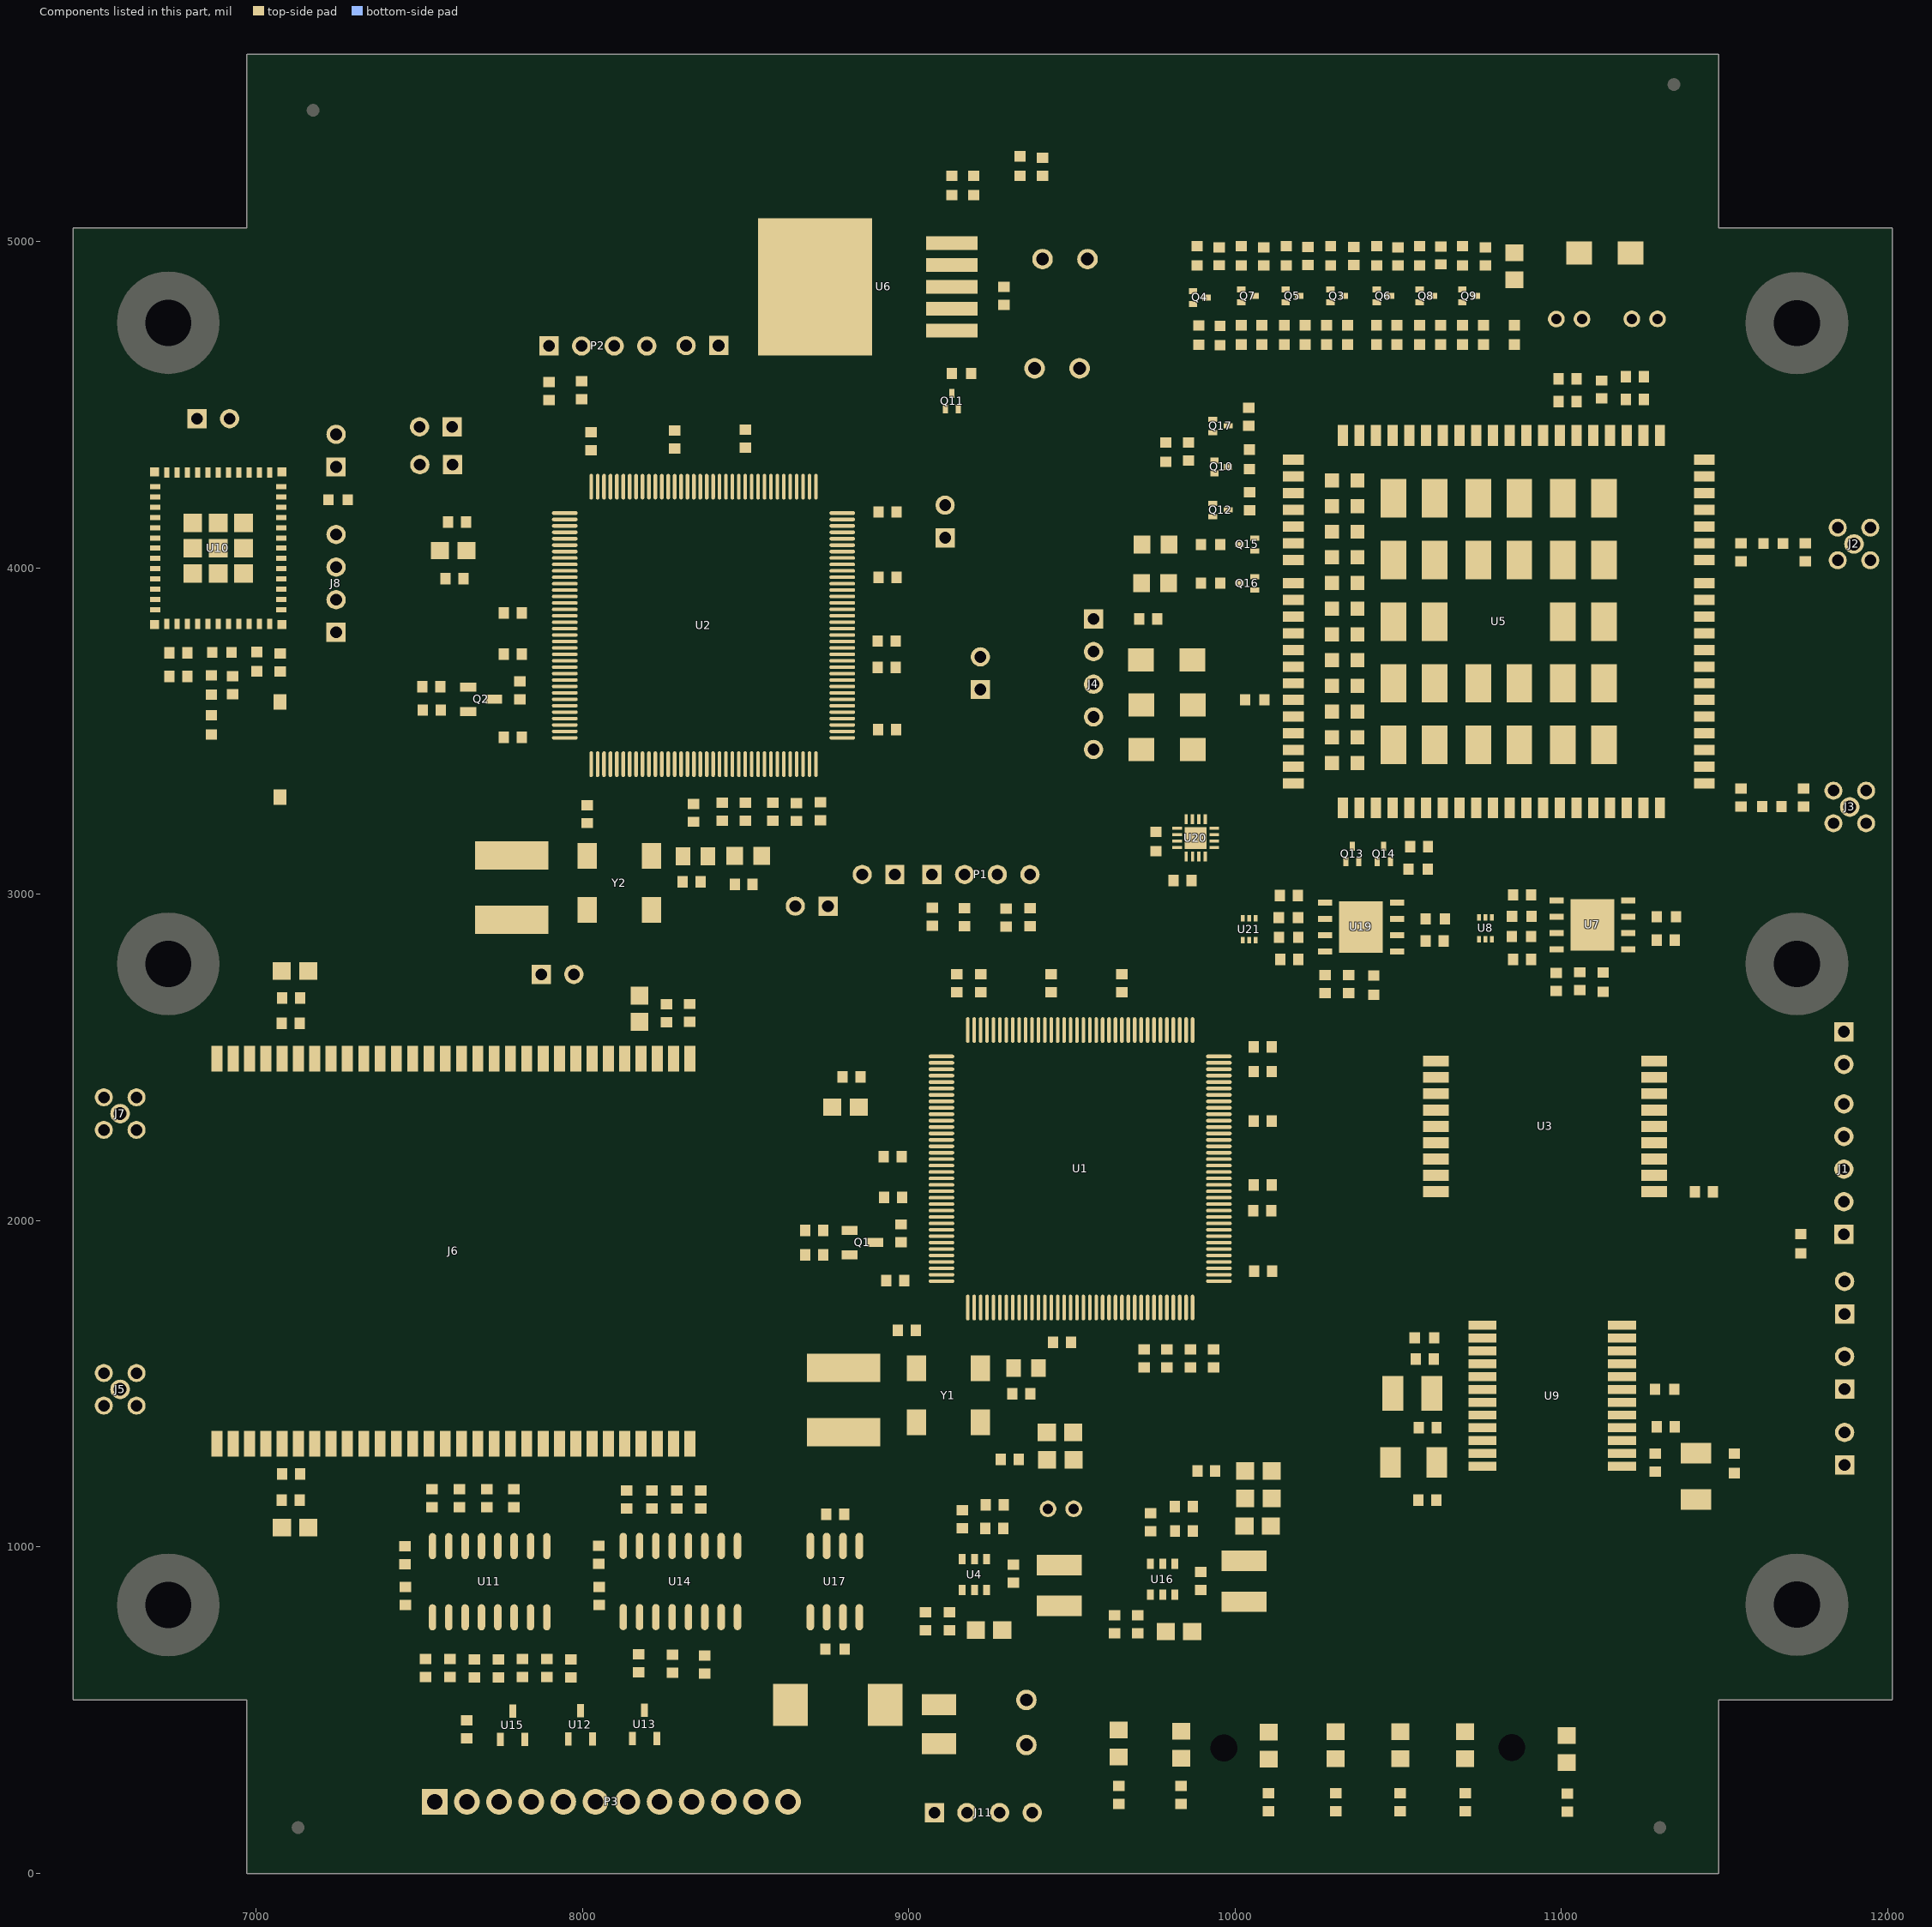
[diagram p0: the components of this part, seen from the top]
# Altium PCB MISC86294.PcbDoc (part 8 of 8)
Units mil, origin at the board's own origin, x right, y up, seen from the top; angles counter-clockwise.
Board outline 5574.84 x 5574.84 mil, 4 copper layers (Top, GND02, PWR03, Bottom), stack 23.756 mil thick; 313 components, 311 nets, 1350 pads, 1701 vias.

## Silkscreen, mask and mechanical layers (free items; w line width, h text height)
Top Overlay:
  text "VBAT" at 9471,5190 h50
  text "WIFI" at 6754,4361 h50 r90
  text "VBAT" at 9377,3834 h50
  text "GND" at 9381,3727 h50
  text "4G" at 11766,3667 h50
  text "KEY" at 9391,3627 h50
  text "RXD" at 9394,3533 h50
  text "TXD" at 9391,3430 h50
  text "SSC" at 11480,2421 h50
  text "RX" at 11723,2342 h50
  text "TX" at 11721,2239 h50
  text "RST" at 11710,2140 h50
  text "GND" at 11707,2043 h50
  text "3.3V" at 11709,1995 h50
  text "GPS" at 6506,1893 h50
  text "VDD_3.3V" at 9804,1298 h50
  text "VDD_5V" at 8929,1229 h50
  text "VDD_IN" at 8938,253 h50
  text "GND" at 9129,251 h50
  text "5V" at 9252,248 h50
  text "3.3V" at 9341,248 h50
  text "RX0" at 8033,44 h50 r90
  text "TX1" at 7750,40 h50 r90
  text "TX0" at 7948,40 h50 r90
  text "RX1" at 7847,39 h50 r90
  text "VCC" at 7555,27 h50 r90
  text "GND" at 7665,27 h50 r90
  text "POWER" at 9098,16 h50
  text "BOO0" at 8647,10 h50 r90
  text "TX232" at 8150,6 h50 r90
  text "BOO1" at 8545,6 h50 r90
  text "CANL" at 8443,5 h50 r90
  text "RX232" at 8242,2 h50 r90
  text "CANH" at 8346,2 h50 r90
Mechanical 1:
  circle w3.94: c11722.41,2786.87 r68.9
  circle w3.94: c11722.41,822.3 r68.9
  circle w3.94: c11722.41,4751.44 r68.9
  circle w3.94: c6730.28,2786.87 r68.9
  circle w3.94: c6730.28,822.3 r68.9
  circle w3.94: c6730.28,4751.44 r68.9
  lines w0.5: 8116.83,504.61 7329.43,504.61 ; 7329.43,504.61 7329.43,110.91 8904.23,110.91 8904.23,504.61 ; 7329.43,504.61 8904.23,504.61 ; 7329.43,504.61 8904.23,504.61
  lines w3.94: 6972.4,5178.61 11480.28,5178.61 ; 9226.34,1.44 9226.34,5572.31 ; 10005.44,384.29 10808.59,385.19 ; 10406.74,634.2 10407.45,1.44 ; 10607.28,499.14 10607.54,270.8 ; 9920.35,533.47 9920.91,38.15 10911.54,39.26 10910.99,534.58 9920.35,533.47 ; 9926.72,364.52 ccw(c9966.09,364.57) 10005.46,364.61 10005.42,403.98 ccw(c9966.05,403.94) 9926.68,403.89 9926.72,364.52 ; 10076.77,498.55 10135.83,498.61 10135.9,429.72 10076.85,429.65 10076.77,498.55 ; 10076.95,339.1 10077.03,270.2 10136.08,270.27 10136,339.17 10076.95,339.1 ; 10277.17,498.77 10336.22,498.84 10336.3,429.94 10277.24,429.87 10277.17,498.77 ; 10277.34,339.32 10336.4,339.39 10336.48,270.49 10277.42,270.43 10277.34,339.32 ; 10477.56,499 10536.61,499.06 10536.69,430.16 10477.63,430.1 10477.56,499 ; 10477.74,339.55 10477.81,270.65 10536.87,270.72 10536.79,339.61 10477.74,339.55 ; 10677.95,499.22 10737.01,499.29 10737.08,430.39 10678.03,430.32 10677.95,499.22 ; 10678.13,339.77 10678.21,270.87 10737.26,270.94 10737.18,339.84 10678.13,339.77 ; 10808.57,404.88 cw(c10847.94,404.92) 10887.31,404.97 10887.35,365.6 cw(c10847.98,365.55) 10808.61,365.51 10808.57,404.88